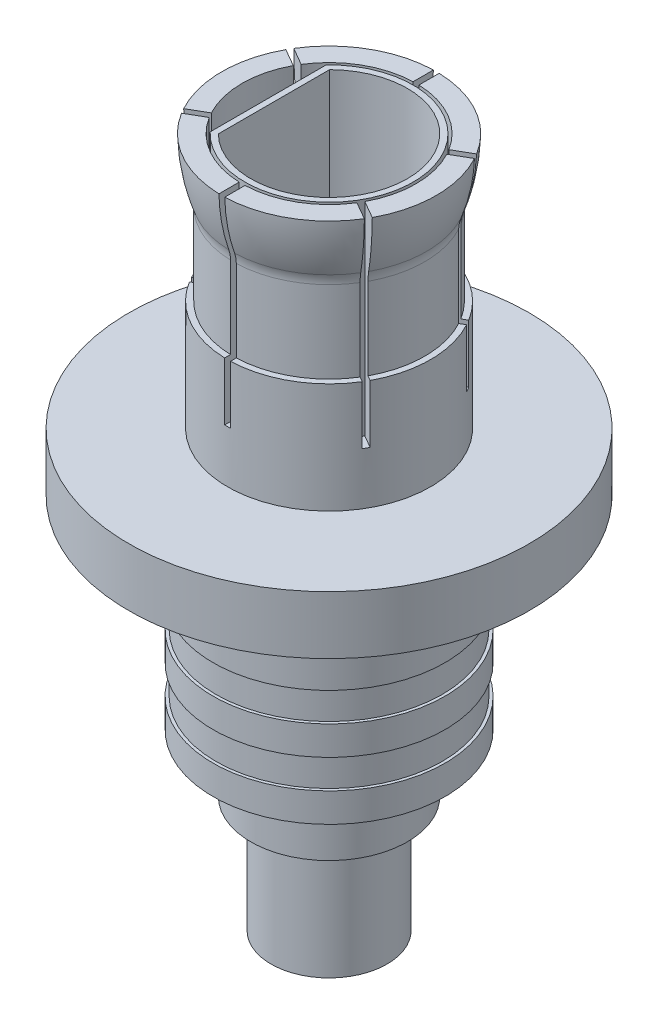
from build123d import *

# Parameters (mm, degrees)
SKETCH2_W           = 0.1
SKETCH2_H           = 4.53654667
CUT_EXTRUDE1_DEPTH  = 3.5
CIRPATTERN1_COUNT   = 3
BOSS_EXTRUDE1_DEPTH = 6
CUT_EXTRUDE2_DEPTH  = 5.9
SKETCH7_R           = 0.565
CUT_EXTRUDE3_DEPTH  = 2


with BuildPart() as part:
    # Sketch1 → Revolve1 (revolve)
    with BuildSketch(Plane.XY, mode=Mode.PRIVATE) as revolve1_sk:
        with BuildLine():
            Line((-1.35, 0), (-1.35, 1))
            Line((-1.35, 1), (-2, 1))
            Line((-2, 1), (-2, 1.5))
            Line((-2, 1.5), (-1.95, 1.5))
            Line((-1.95, 1.5), (-1.95, 2))
            Line((-1.95, 2), (-2, 2))
            Line((-2, 2), (-2, 2.5))
            Line((-2, 2.5), (-1.95, 2.5))
            Line((-1.95, 2.5), (-1.95, 3))
            Line((-1.95, 3), (-2, 3))
            Line((-2, 3), (-2, 3.5))
            Line((-2, 3.5), (-1.95, 3.5))
            Line((-1.95, 3.5), (-1.95, 4))
            Line((-1.95, 4), (-2, 4))
            Line((-2, 4), (-2, 4.5))
            Line((-2, 4.5), (-3.45, 4.5))
            Line((-3.45, 4.5), (-3.45, 5.5))
            Line((-3.45, 5.5), (-1.75, 5.5))
            Line((-1.75, 5.5), (-1.75, 7.4))
            Line((-1.75, 7.4), (-1.65, 7.4))
            Line((-1.65, 7.4), (-1.65, 8.810842582))
            ThreePointArc((-1.65, 8.810842582), (-1.65719462, 8.895358008), (-1.678571429, 8.977441208))
            ThreePointArc((-1.678571429, 8.977441208), (-1.800077526, 9.432016823), (-1.849010824, 9.9))
            Line((-1.849010824, 9.9), (-1.5, 9.9))
            Line((-1.5, 9.9), (-1.5, 3.9))
            Line((-1.5, 3.9), (-0.6, 3.9))
            Line((-0.6, 3.9), (-0.6, -2))
            Line((-0.6, -2), (-1, -2))
            Line((-1, -2), (-1, 0))
            Line((-1, 0), (-1.35, 0))
        make_face()
    revolve(revolve1_sk.sketch.rotate(Axis((0, 0, 0), (0, 1, 0)), 270), axis=Axis((0, 0, 0), (0, 1, 0)))

    # Sketch2 → Cut-Extrude1 (cut)
    with BuildSketch(Plane(origin=(0, 9.9, 0), x_dir=(1, 0, 0), z_dir=(0, 1, 0))):
        Rectangle(SKETCH2_W, SKETCH2_H)
    cut_extrude1 = extrude(amount=-CUT_EXTRUDE1_DEPTH, mode=Mode.SUBTRACT)

    # CirPattern1: Cut-Extrude1 ×3 about axis
    cirpattern1_axis = Axis((0, 0, 0), (0, 1, 0))
    for i in range(1, CIRPATTERN1_COUNT):
        add(cut_extrude1.rotate(cirpattern1_axis, i * 360 / CIRPATTERN1_COUNT), mode=Mode.SUBTRACT)

    # Sketch5 → Boss-Extrude1 (add)
    with BuildSketch(Plane(origin=(0, 3.9, 0), x_dir=(1, 0, 0), z_dir=(0, 1, 0))):
        with BuildLine():
            Line((-1.05, 1), (-1.05, -1))
            ThreePointArc((-1.05, -1), (1.45, 0), (-1.05, 1))
        make_face()
    extrude(amount=BOSS_EXTRUDE1_DEPTH)

    # Sketch6 → Cut-Extrude2 (cut)
    with BuildSketch(Plane(origin=(0, 9.9, 0), x_dir=(1, 0, 0), z_dir=(0, 1, 0))):
        with BuildLine():
            Line((-0.95, 0.959166305), (-0.95, -0.959166305))
            ThreePointArc((-0.95, -0.959166305), (1.35, 0), (-0.95, 0.959166305))
        make_face()
    extrude(amount=-CUT_EXTRUDE2_DEPTH, mode=Mode.SUBTRACT)

    # Sketch7 → Cut-Extrude3 (cut)
    with BuildSketch(Plane(origin=(0, 4, 0), x_dir=(1, 0, 0), z_dir=(0, 1, 0))):
        with Locations(Location((0, 0, 0), (0, 0, 270))):
            Circle(SKETCH7_R)
    extrude(amount=-CUT_EXTRUDE3_DEPTH, mode=Mode.SUBTRACT)


solid = part.part
